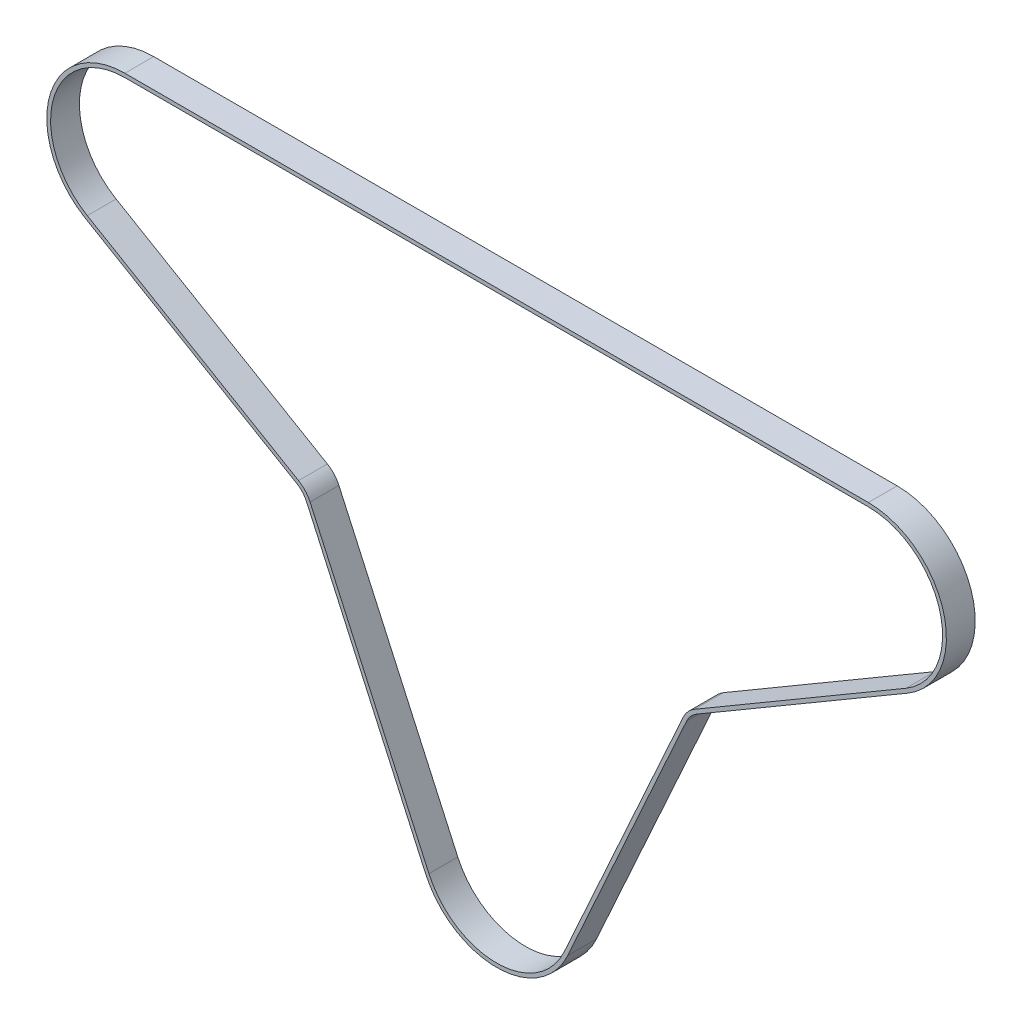
SolidWorks part; units mm, degrees
ref_plane "前视基准面" through (0, 0, 0) normal (0, 0, 1) x (1, 0, 0)
ref_plane "上视基准面" through (0, 0, 0) normal (0, 1, 0) x (1, 0, 0)
ref_plane "右视基准面" through (0, 0, 0) normal (1, 0, 0) x (0, 0, -1)
sketch "草图2" plane through (0, 0, 0) normal (0, 0, 1) x (1, 0, 0)
  line L0 (0, 0) -> (1, 0) construction
  line L1 (0, 0) -> (0, 1) construction
  line L2 (-91.435, -41.422) -> (-248.1189, 304.4428)
  line L3 (-262.3022, 320.1958) -> (-540.7572, 483.3983)
  line L4 (-490, 670.38) -> (490, 670.38)
  line L5 (540.7572, 483.3983) -> (262.3022, 320.1958)
  line L6 (248.1189, 304.4428) -> (91.435, -41.422)
  arc A0 (91.435, -41.422) -> (-91.435, -41.422) centre (0, 0) cw
  arc A1 (-248.1189, 304.4428) -> (-262.3022, 320.1958) centre (-280, 290) ccw
  arc A2 (-540.7572, 483.3983) -> (-490, 670.38) centre (-490, 570) cw
  arc A3 (490, 670.38) -> (540.7572, 483.3983) centre (490, 570) cw
  arc A4 (262.3022, 320.1958) -> (248.1189, 304.4428) centre (280, 290) ccw
extrude "拉伸-薄壁1" add sketch "草图2" along normal mid plane 38 thin thin type mid plane wall 5
